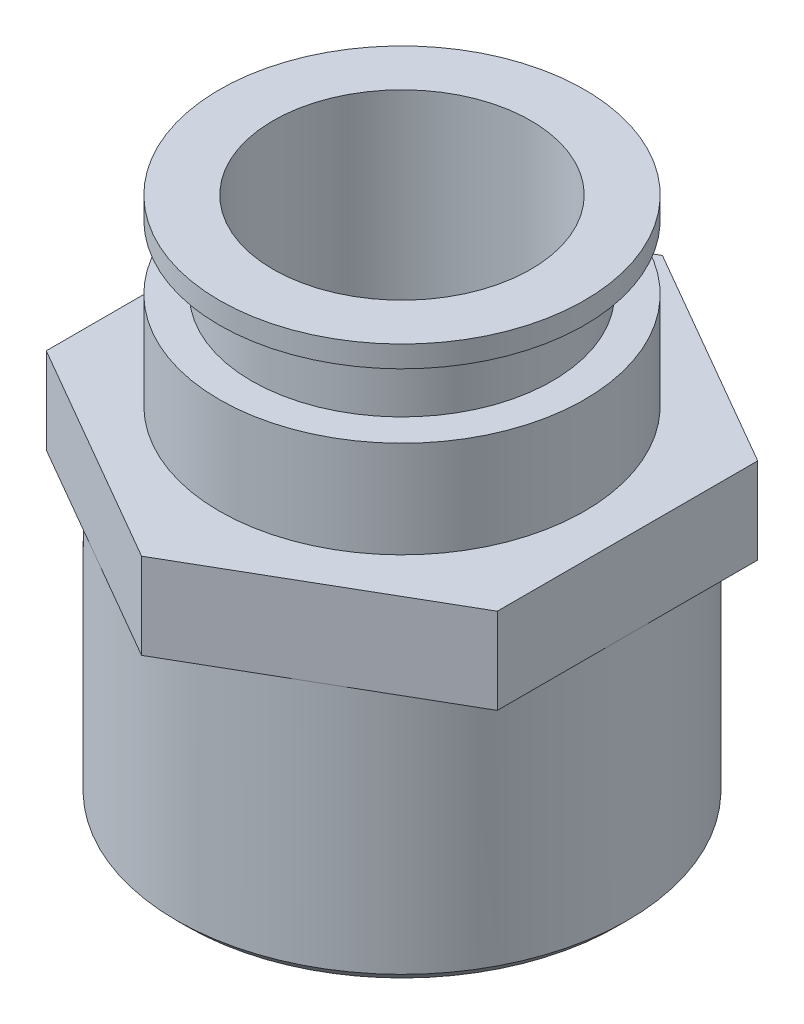
from build123d import *

# Parameters (mm, degrees)
SKETCH2_R           = 10.5
BOSS_EXTRUDE1_DEPTH = 12
BOSS_EXTRUDE2_DEPTH = 4
SKETCH4_R           = 8.5
BOSS_EXTRUDE3_DEPTH = 4.5
SKETCH5_R           = 7
BOSS_EXTRUDE4_DEPTH = 3
SKETCH7_R           = 8.5
BOSS_EXTRUDE5_DEPTH = 1
CHAMFER1_SIZE       = 0.5
SKETCH9_R           = 6
CUT_EXTRUDE1_DEPTH  = 11
SKETCH8_R           = 5
CUT_EXTRUDE2_DEPTH  = 30.283100929


with BuildPart() as part:
    # Sketch2 → Boss-Extrude1 (new body)
    with BuildSketch(Plane(origin=(0, 0, 0), x_dir=(1, 0, 0), z_dir=(0, 1, 0))):
        with Locations(Location((0, 0, 0), (0, 0, 270))):
            Circle(SKETCH2_R)
    extrude(amount=BOSS_EXTRUDE1_DEPTH)

    # Sketch3 → Boss-Extrude2 (add)
    with BuildSketch(Plane(origin=(0, 12, 0), x_dir=(1, 0, 0), z_dir=(0, 1, 0))):
        Polygon((10.5, -6.062177826), (10.5, 6.062177826), (0, 12.124355653), (-10.5, 6.062177826), (-10.5, -6.062177826), (0, -12.124355653), align=None)
    extrude(amount=BOSS_EXTRUDE2_DEPTH)

    # Sketch4 → Boss-Extrude3 (add)
    with BuildSketch(Plane(origin=(0, 16, 0), x_dir=(1, 0, 0), z_dir=(0, 1, 0))):
        with Locations(Location((0, 0, 0), (0, 0, 270))):
            Circle(SKETCH4_R)
    extrude(amount=BOSS_EXTRUDE3_DEPTH)

    # Sketch5 → Boss-Extrude4 (add)
    with BuildSketch(Plane(origin=(0, 20.5, 0), x_dir=(1, 0, 0), z_dir=(0, 1, 0))):
        with Locations(Location((0, 0, 0), (0, 0, 270))):
            Circle(SKETCH5_R)
    extrude(amount=BOSS_EXTRUDE4_DEPTH)

    # Sketch7 → Boss-Extrude5 (add)
    with BuildSketch(Plane(origin=(0, 23.5, 0), x_dir=(1, 0, 0), z_dir=(0, 1, 0))):
        with Locations(Location((0, 0, 0), (0, 0, 270))):
            Circle(SKETCH7_R)
    extrude(amount=BOSS_EXTRUDE5_DEPTH)

    # Chamfer1
    chamfer1_edges = [part.edges().sort_by_distance(p)[0] for p in [
        (0, 0, -10.5),
    ]]
    chamfer(chamfer1_edges, length=CHAMFER1_SIZE)

    # Sketch9 → Cut-Extrude1 (cut)
    with BuildSketch(Plane(origin=(0, 24.5, 0), x_dir=(1, 0, 0), z_dir=(0, 1, 0))):
        with Locations(Location((0, 0, 0), (0, 0, 270))):
            Circle(SKETCH9_R)
    extrude(amount=-CUT_EXTRUDE1_DEPTH, mode=Mode.SUBTRACT)

    # Sketch8 → Cut-Extrude2 (cut, through all)
    with BuildSketch(Plane.XZ):
        with Locations(Location((0, 0, 0), (0, 0, 270))):
            Circle(SKETCH8_R)
    extrude(amount=-CUT_EXTRUDE2_DEPTH, mode=Mode.SUBTRACT)


solid = part.part
